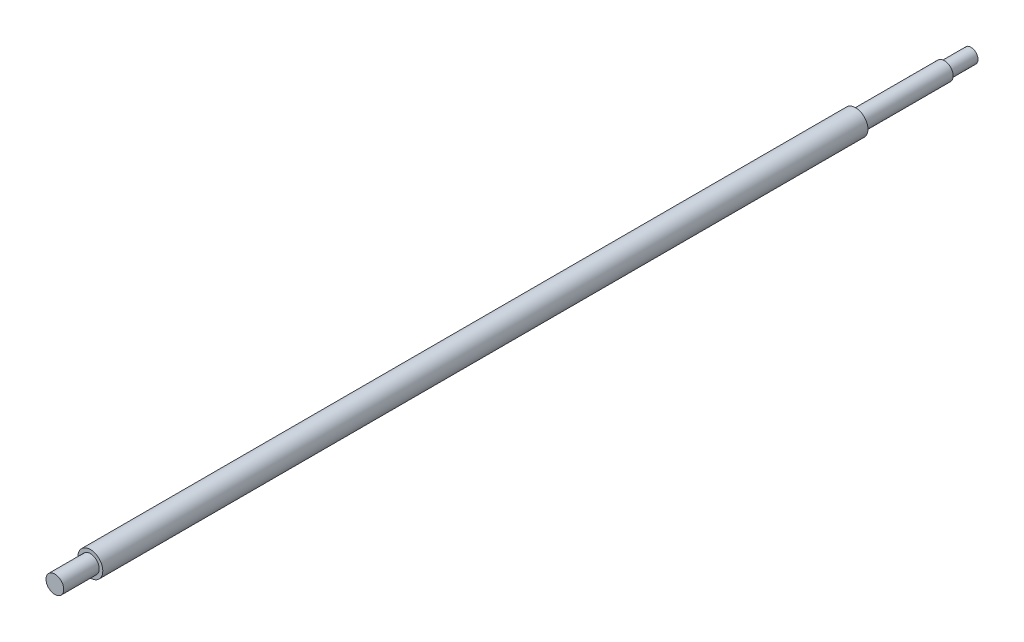
SolidWorks part; units mm, degrees
ref_plane "Front Plane" through (0, 0, 0) normal (0, 0, 1) x (1, 0, 0)
ref_plane "Top Plane" through (0, 0, 0) normal (0, 1, 0) x (1, 0, 0)
ref_plane "Right Plane" through (0, 0, 0) normal (1, 0, 0) x (0, 0, -1)
other "Configuration Table"
sketch "Sketch1" plane through (0, 0, 0) normal (0, 0, 1) x (1, 0, 0)
  circle A0 centre (0, 0) radius 7
  dimension "D1" = 14
extrude "Boss-Extrude1" add sketch "Sketch1" along normal blind 431
sketch "Sketch2" plane through (0, 0, 431) normal (0, 0, 1) x (1, 0, 0)
  circle A0 centre (0, 0) radius 5
  dimension "D1" = 10
extrude "Boss-Extrude2" add sketch "Sketch2" along normal blind 20
sketch "Sketch3" plane through (0, 0, 0) normal (0, 0, -1) x (-1, 0, 0)
  circle A0 centre (0, 0) radius 5
  dimension "D1" = 10
extrude "Boss-Extrude3" add sketch "Sketch3" along normal blind 50
sketch "Sketch4" plane through (0, 0, -50) normal (0, 0, -1) x (-1, 0, 0)
  circle A0 centre (0, 0) radius 4
  dimension "D1" = 8
extrude "Boss-Extrude4" add sketch "Sketch4" along normal blind 15
